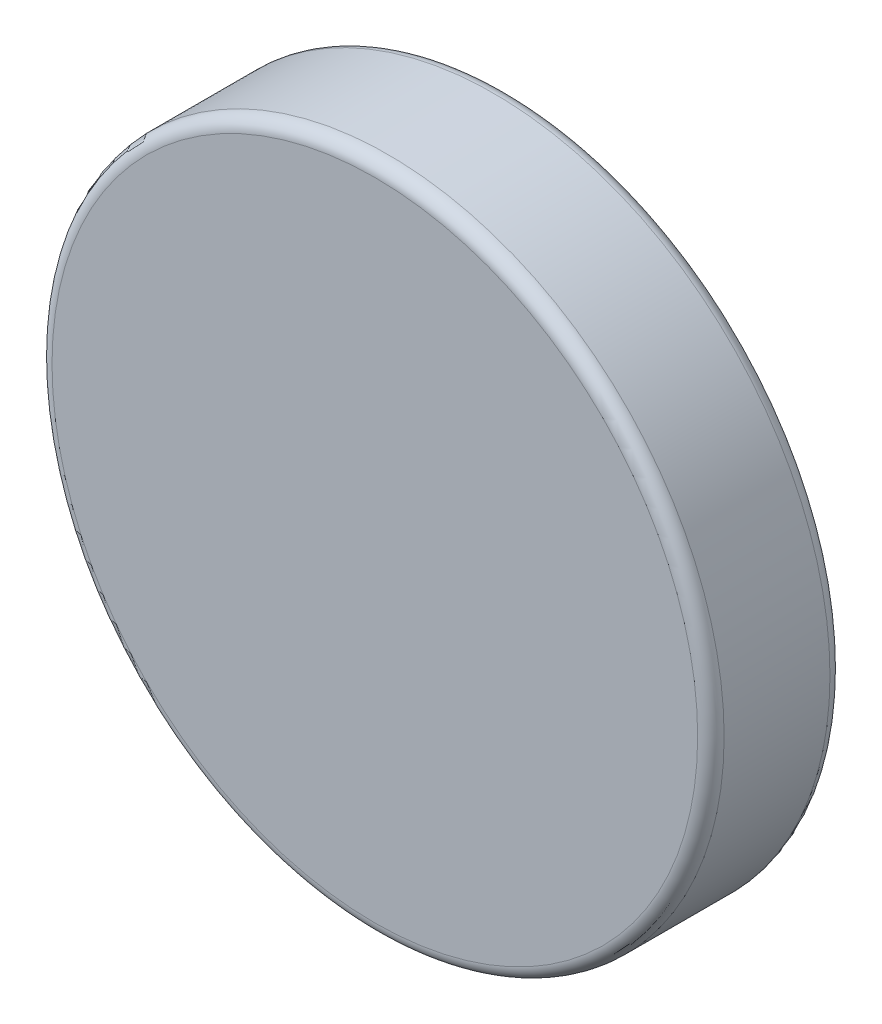
from build123d import *

# Parameters (mm, degrees)
SKETCH1_R           = 12.7
BOSS_EXTRUDE1_DEPTH = 5
FILLET1_R           = 0.5


with BuildPart() as part:
    # Sketch1 → Boss-Extrude1 (new body)
    with BuildSketch(Plane.XY):
        Circle(SKETCH1_R)
    extrude(amount=BOSS_EXTRUDE1_DEPTH)

    # Fillet1
    fillet1_edges = [part.edges().sort_by_distance(p)[0] for p in [
        (-12.7, 0, 0),
        (-12.7, 0, 5),
    ]]
    fillet(fillet1_edges, radius=FILLET1_R)


solid = part.part
